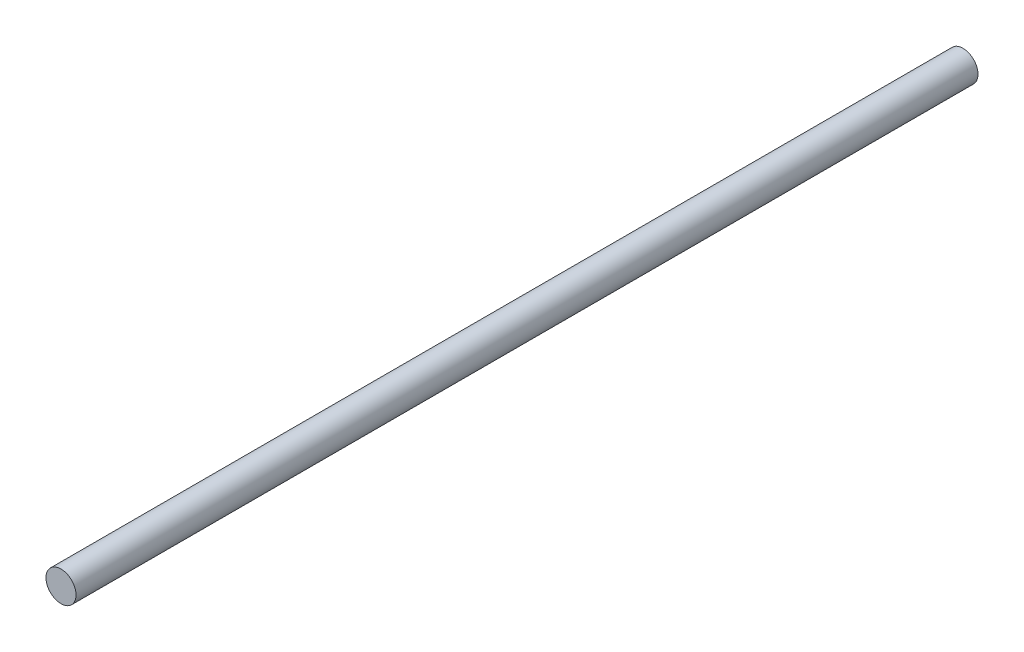
from build123d import *

# Parameters (mm, degrees)
SKETCH1_R           = 1
BOSS_EXTRUDE1_DEPTH = 60


with BuildPart() as part:
    # Sketch1 → Boss-Extrude1 (new body)
    with BuildSketch(Plane.XY):
        Circle(SKETCH1_R)
    extrude(amount=BOSS_EXTRUDE1_DEPTH)


solid = part.part
